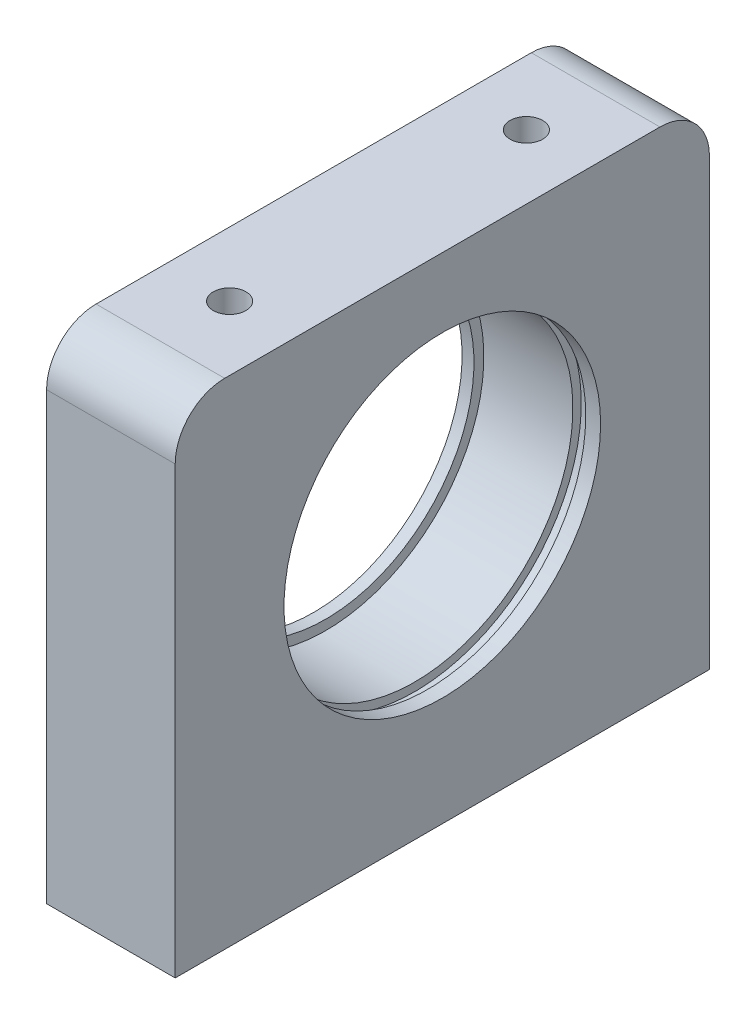
SolidWorks part; units mm, degrees
material "6061 合金"
ref_plane "前视" through (0, 0, 0) normal (0, 0, 1) x (1, 0, 0)
ref_plane "上视" through (0, 0, 0) normal (0, 1, 0) x (1, 0, 0)
ref_plane "右视" through (0, 0, 0) normal (1, 0, 0) x (0, 0, -1)
sketch "草图1" plane through (0, 0, 0) normal (0, 0, 1) x (1, 0, 0)
  line L0 (0, 0) -> (0, 50)
  line L1 (0, 0) -> (90, 0)
  dimension "D1" = 50
  dimension "D2" = 90
extrude "拉伸-薄壁1" add sketch "草图1" along normal mid plane 54 thin thin type one direction wall 13
sketch "草图2" plane through (0, 0, 0) normal (1, 0, 0) x (0, 0, -1)
  line L0 (0, 0) -> (0, 27) construction
  line L1 (-27, -13) -> (27, -13) construction
  circle A0 centre (0, 27) radius 16
  dimension "D1" = 32
  dimension "D2" = 40
extrude "切除-拉伸1" cut sketch "草图2" against normal through all
sketch "草图3" plane through (-13, 0, 0) normal (-1, 0, 0) x (0, 0, 1)
  circle A0 centre (0, 27) radius 15
  circle A1 centre (0, 27) radius 16 construction
  circle A2 centre (0, 27) radius 16
  dimension "D1" = 30
extrude "凸台-拉伸1" add sketch "草图3" against normal blind 1.2
sketch "草图4" plane through (0, 0, 0) normal (0, 0, 1) x (1, 0, 0)
  line L0 (-2.8, 43) -> (-2.8, 43.85)
  line L1 (0, 43) -> (-11.8, 43) construction
  line L2 (-2.8, 43.85) -> (-1.5, 43.85)
  line L3 (-1.5, 43.85) -> (-1.5, 43)
  line L4 (-1.5, 43) -> (-2.8, 43)
  line L5 (-11.8, 27) -> (4.6946, 27) construction
  line L6 (-11.8, 11) -> (-11.8, 43) construction
  dimension "D1" = 1.3
  dimension "D2" = 33.7
  dimension "D3" = 9
revolve "切除-旋转1" cut sketch "草图4" angle 360 about L5
sketch "草图5" plane through (0, 0, 0) normal (0, 1, 0) x (1, 0, 0)
  line L0 (90, -27) -> (90, 27) construction
  line L1 (-13, -52.5) -> (90, -52.5)
  line L2 (-13, -52.5) -> (-13, 52.5)
  line L3 (-13, 52.5) -> (90, 52.5)
  line L4 (90, -52.5) -> (90, 52.5)
  line L5 (-13, -52.5) -> (90, 52.5) construction
  line L6 (-13, 52.5) -> (90, -52.5) construction
  line L7 (0, 0) -> (70.3449, 0) construction
  line L8 (0, -27) -> (0, 27) construction
  line L9 (-13, -27) -> (-13, 27) construction
  point P0 (38.5, 0)
  dimension "D2" = 105
extrude "凸台-拉伸2" add sketch "草图5" against normal up to surface (13 mm away) up to face at (38.5, -13, 0)
fillet "圆角1" radius 5 6 edges at (-13, -6.5, -52.5) (90, -6.5, -52.5) (90, -6.5, 52.5) (-13, -6.5, 52.5) (-6.5, 50, -27) (-6.5, 50, 27)
sketch "草图6" plane through (0, -13, 0) normal (0, -1, 0) x (1, 0, 0)
  line L4 (-13, 47.5) -> (-13, -47.5)
  line L5 (-8, -52.5) -> (85, -52.5)
  line L6 (90, -47.5) -> (90, 47.5)
  line L7 (85, 52.5) -> (-8, 52.5)
  line L8 (-13, 47.5) -> (-13, -47.5)
  line L9 (-8, -52.5) -> (85, -52.5)
  line L10 (90, -47.5) -> (90, 47.5)
  line L11 (85, 52.5) -> (-8, 52.5)
  arc A4 (-13, -47.5) -> (-8, -52.5) centre (-8, -47.5) ccw
  arc A5 (85, -52.5) -> (90, -47.5) centre (85, -47.5) ccw
  arc A6 (90, 47.5) -> (85, 52.5) centre (85, 47.5) ccw
  arc A7 (-8, 52.5) -> (-13, 47.5) centre (-8, 47.5) ccw
  arc A8 (-13, -47.5) -> (-8, -52.5) centre (-8, -47.5) ccw
  arc A9 (85, -52.5) -> (90, -47.5) centre (85, -47.5) ccw
  arc A10 (90, 47.5) -> (85, 52.5) centre (85, 47.5) ccw
  arc A11 (-8, 52.5) -> (-13, 47.5) centre (-8, 47.5) ccw
  dimension "D1" = 0
extrude "切除-拉伸2" cut sketch "草图6" against normal blind 13
sketch "草图7" plane through (0, 0, 0) normal (0, -1, 0) x (1, 0, 0)
  line L0 (-6.5, 27) -> (-6.5, -27) construction
  line L1 (0, 27) -> (-13, 27) construction
  line L2 (0, -27) -> (-13, -27) construction
  line L3 (0, 0) -> (-6.5, 0) construction
  point P9 (-6.5, 20)
  point P10 (-6.5, -20)
  dimension "D1" = 40
hole_wizard "M5 螺纹孔1" positions "3D草图1" profile "草图8" tap size "M5" standard "GB"
sketch3d "3D草图1"
  point P0 (-6.5, 0, 20)
  point P3 (-6.5, 0, -20)
sketch "草图8" plane through (-6.5, 0, 20) normal (1, 0, 0) x (0, 0, -1)
  line L0 (0, 0) -> (0, 13.6618)
  line L1 (0, 13.6618) -> (2.1, 12.4)
  line L2 (2.1, 12.4) -> (2.1, 0)
  line L5 (2.1, 0) -> (0, 0)
  line L10 (0, 13.6618) -> (-2.1, 12.4) construction
  line L11 (0, -6.35) -> (0, 107.95) construction
  dimension "螺纹孔钻头直径" = 4.2
  dimension "螺纹孔钻头深度" = 12.4
  dimension "导头角度" = 118
cosmetic thread "孔螺蚊线1" parameters "D1"=10, "D2"=5
cosmetic thread "孔螺蚊线2" parameters "D1"=10, "D2"=5
sketch "草图9" plane through (0, 50, 0) normal (0, 1, 0) x (1, 0, 0)
  line L0 (-6.5, 22) -> (-6.5, -22) construction
  line L2 (-13, -22) -> (0, -22) construction
  line L3 (0, 0) -> (-6.5, 0) construction
  point P2 (-6.5, 15)
  point P3 (-6.5, -15)
  dimension "D1" = 30
hole_wizard "M4 螺纹孔1" positions "3D草图2" profile "草图10" tap size "M4" standard "GB"
sketch3d "3D草图2"
  point P0 (-6.5, 50, -15)
  point P3 (-6.5, 50, 15)
sketch "草图10" plane through (-6.5, 50, -15) normal (1, 0, 0) x (0, 0, 1)
  line L0 (0, 0) -> (0, 11.0914)
  line L1 (0, 11.0914) -> (1.65, 10.1)
  line L2 (1.65, 10.1) -> (1.65, 0)
  line L5 (1.65, 0) -> (0, 0)
  line L10 (0, 11.0914) -> (-1.65, 10.1) construction
  line L11 (0, -6.35) -> (0, 107.95) construction
  dimension "螺纹孔钻头直径" = 3.3
  dimension "螺纹孔钻头深度" = 10.1
  dimension "导头角度" = 118
cosmetic thread "孔螺蚊线3" parameters "D1"=8, "D2"=4
cosmetic thread "孔螺蚊线4" parameters "D1"=8, "D2"=4
